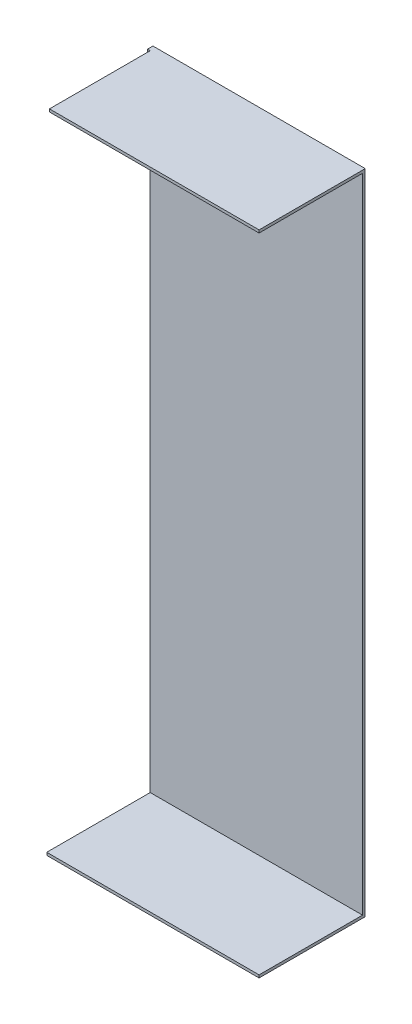
from build123d import *

# Parameters (mm, degrees)
SKETCH1_W           = 77
SKETCH1_H           = 238
BOSS_EXTRUDE1_DEPTH = 1
SKETCH2_W           = 77
SKETCH2_H           = 1
BOSS_EXTRUDE2_DEPTH = 38
BOSS_EXTRUDE3_DEPTH = 1


with BuildPart() as part:
    # Sketch1 → Boss-Extrude1 (new body)
    with BuildSketch(Plane.XY):
        Rectangle(SKETCH1_W, SKETCH1_H)
    extrude(amount=BOSS_EXTRUDE1_DEPTH)

    # Sketch2 → Boss-Extrude2 (add)
    with BuildSketch(Plane.XY.offset(1)):
        with Locations((0, 118.5)):
            Rectangle(SKETCH2_W, SKETCH2_H)
        with Locations((0, -118.5)):
            Rectangle(SKETCH2_W, SKETCH2_H)
    extrude(amount=BOSS_EXTRUDE2_DEPTH)

    # Sketch3 → Boss-Extrude3 (add)
    with BuildSketch(Plane.ZY.offset(38.5)):
        Polygon((2, 119), (0, 119), (0, -119), (39, -119), (39, -118), (1, -118), (1, 118), (2, 118), align=None)
    extrude(amount=BOSS_EXTRUDE3_DEPTH)


solid = part.part
